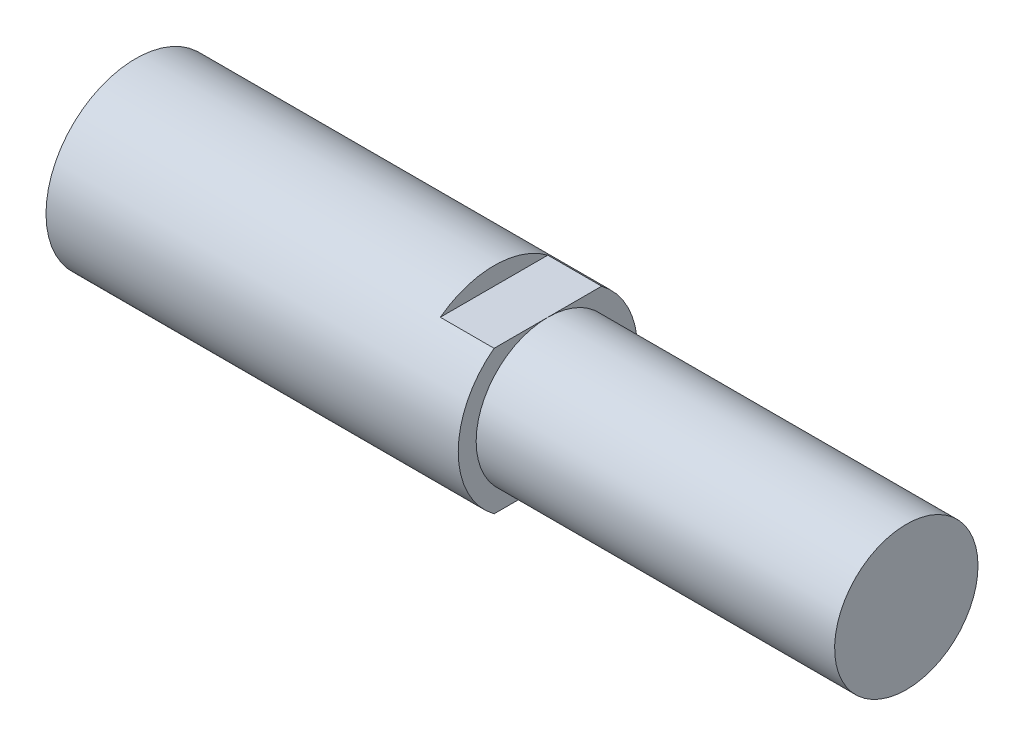
SolidWorks part; units mm, degrees
ref_plane "前视基准面" through (0, 0, 0) normal (0, 0, 1) x (1, 0, 0)
ref_plane "上视基准面" through (0, 0, 0) normal (0, 1, 0) x (1, 0, 0)
ref_plane "右视基准面" through (0, 0, 0) normal (1, 0, 0) x (0, 0, -1)
sketch "草图1" plane through (0, 0, 0) normal (1, 0, 0) x (0, 0, -1)
  circle A0 centre (0, 0) radius 4
  dimension "D1" = 8
extrude "凸台-拉伸1" add sketch "草图1" along normal blind 20
sketch "草图2" plane through (0, 0, 0) normal (-1, 0, 0) x (0, 0, 1)
  circle A0 centre (0, 0) radius 5
  dimension "D1" = 10
extrude "凸台-拉伸2" add sketch "草图2" along normal blind 3
sketch "草图3" plane through (-3, 0, 0) normal (-1, 0, 0) x (0, 0, 1)
  line L1 (-7.0869, 4) -> (7.0869, 4)
  line L2 (-7.0869, 4) -> (-7.0869, -4)
  line L3 (-7.0869, -4) -> (7.0869, -4)
  line L4 (7.0869, 4) -> (7.0869, -4)
  line L5 (-7.0869, 4) -> (7.0869, -4) construction
  line L6 (-7.0869, -4) -> (7.0869, 4) construction
  point P0 (0, 0)
  dimension "D1" = 8
extrude "切除-拉伸1" cut sketch "草图3" against normal through all flip side to cut
sketch "草图4" plane through (-3, 0, 0) normal (-1, 0, 0) x (0, 0, 1)
  circle A0 centre (0, 0) radius 5
  dimension "D1" = 10
extrude "凸台-拉伸3" add sketch "草图4" along normal blind 20
